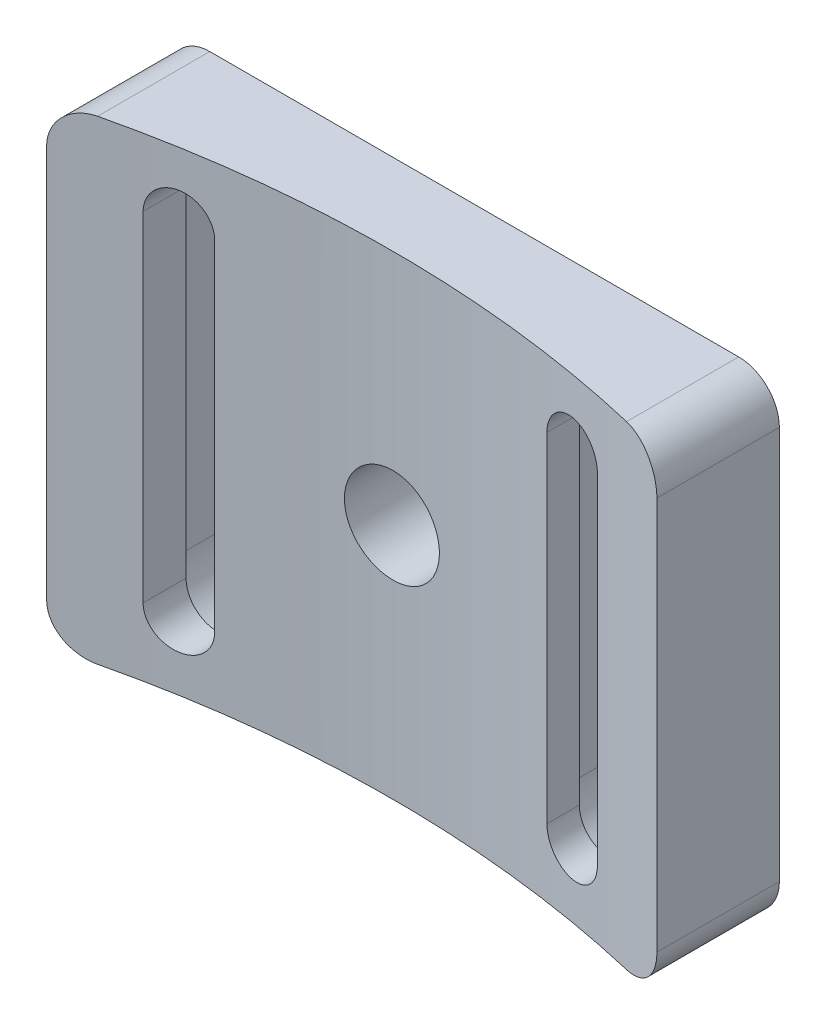
SolidWorks part; units mm, degrees
ref_plane "Front Plane" through (0, 0, 0) normal (0, 0, 1) x (1, 0, 0)
ref_plane "Top Plane" through (0, 0, 0) normal (0, 1, 0) x (1, 0, 0)
ref_plane "Right Plane" through (0, 0, 0) normal (1, 0, 0) x (0, 0, -1)
sketch "Sketch1" plane through (0, 0, 0) normal (0, 1, 0) x (1, 0, 0)
  line L0 (-22.5, 81.968) -> (-22.5, 91)
  line L1 (-22.5, 91) -> (22.5, 91)
  line L2 (22.5, 91) -> (22.5, 81.968)
  line L3 (0, 0) -> (0, 103.5063) construction
  arc A0 (22.5, 81.968) -> (-22.5, 81.968) centre (0, 0) ccw
  dimension "D1" = 170
  dimension "D2" = 45
  dimension "D4" = 91
extrude "Boss-Extrude1" add sketch "Sketch1" along normal blind 35
fillet "Fillet1" radius 3 4 edges at (-22.5, 0, -86.484) (-22.5, 35, -86.484) (22.5, 0, -86.484) (22.5, 35, -86.484)
hole_wizard "M8x1.0 Tapped Hole1" positions "Sketch3" profile "Sketch2" tap size "M8x1.0" standard "GB" end condition through all
sketch "Sketch3" plane through (0, 0, -91) normal (0, 0, -1) x (-1, 0, 0)
  line L0 (-19.5, 35) -> (19.5, 35) construction
  line L1 (-22.5, 32) -> (-22.5, 3) construction
  point P0 (0, 17.5)
  point P3 (0, 35)
  point P6 (-22.5, 17.5)
  dimension "D1" = 0
  dimension "D2" = 0
sketch "Sketch2" plane through (0, 17.5, -91) normal (1, 0, 0) x (0, 1, 0)
  line L0 (0, 0) -> (0, 9.2152)
  line L1 (0, 9.2152) -> (3.5, 9.2152)
  line L2 (3.5, 9.2152) -> (3.5, 0)
  line L5 (3.5, 0) -> (0, 0)
  line L11 (0, -6.35) -> (0, 107.95) construction
  dimension "通孔螺纹孔钻头直径" = 7
  dimension "通孔螺纹孔钻头深度" = 9.2152
cosmetic thread "Cosmetic thread 1" parameters "D2"=8
sketch "Sketch4" plane through (0, 0, -91) normal (0, 0, -1) x (-1, 0, 0)
  line L0 (-14.5, 30) -> (-14.5, 5) construction
  line L1 (-12.25, 30) -> (-12.25, 5)
  line L2 (-16.75, 30) -> (-16.75, 5)
  line L3 (14.5, 30) -> (14.5, 5) construction
  line L4 (16.75, 30) -> (16.75, 5)
  line L5 (12.25, 30) -> (12.25, 5)
  line L10 (0, 0) -> (0, 39.4662) construction
  line L11 (-22.5, 17.5) -> (30.8561, 17.5) construction
  line L12 (-22.5, 32) -> (-22.5, 3) construction
  arc A0 (-12.25, 30) -> (-16.75, 30) centre (-14.5, 30) ccw
  arc A1 (-16.75, 5) -> (-12.25, 5) centre (-14.5, 5) ccw
  arc A2 (16.75, 30) -> (12.25, 30) centre (14.5, 30) ccw
  arc A3 (12.25, 5) -> (16.75, 5) centre (14.5, 5) ccw
  point P2 (-14.5, 17.5)
  point P7 (14.5, 17.5)
  dimension "D5" = 2.25
  dimension "D6" = 2.25
  dimension "D1" = 29
  dimension "D3" = 25
  dimension "D4" = 25
extrude "Cut-Extrude1" cut sketch "Sketch4" against normal through all
sketch "Sketch5" plane through (0, 0, -91) normal (0, 0, -1) x (-1, 0, 0)
  line L0 (-14.5, 30) -> (-14.5, 5) construction
  line L1 (-10.5, 30) -> (-10.5, 5)
  line L2 (-18.5, 30) -> (-18.5, 5)
  line L3 (14.5, 30) -> (14.5, 5) construction
  line L4 (18.5, 30) -> (18.5, 5)
  line L5 (10.5, 30) -> (10.5, 5)
  arc A0 (-10.5, 30) -> (-18.5, 30) centre (-14.5, 30) ccw
  arc A1 (-18.5, 5) -> (-10.5, 5) centre (-14.5, 5) ccw
  arc A2 (18.5, 30) -> (10.5, 30) centre (14.5, 30) ccw
  arc A3 (10.5, 5) -> (18.5, 5) centre (14.5, 5) ccw
  point P2 (-14.5, 17.5)
  point P7 (14.5, 17.5)
  dimension "D1" = 4
  dimension "D2" = 4
extrude "Cut-Extrude2" cut sketch "Sketch5" against normal blind 4.5
